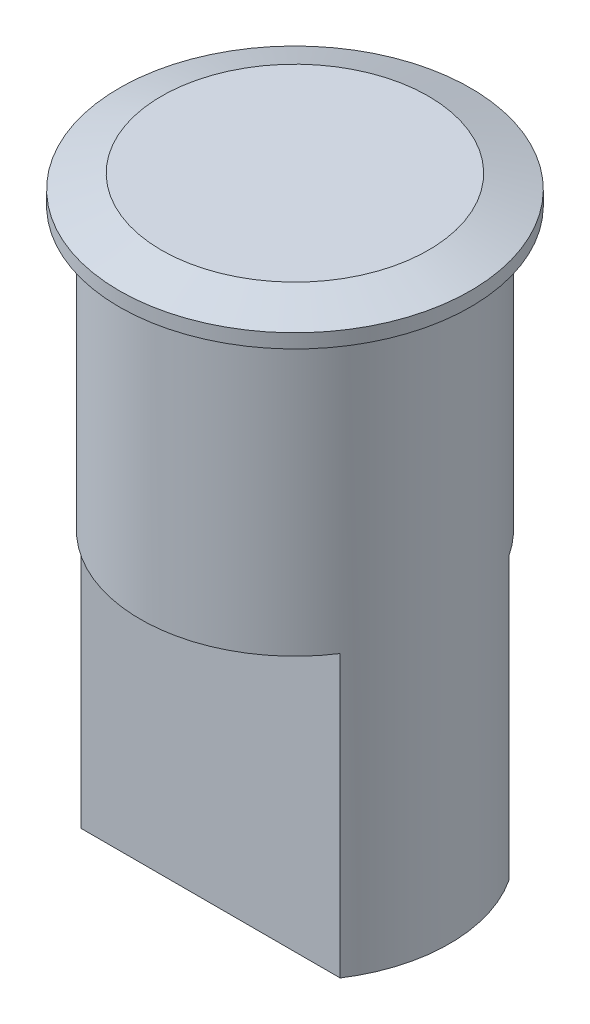
from build123d import *
from build123d.topology import SkipClean

# Parameters (mm, degrees)
SKETCH_1_R      = 11
EXTRUDE_1_DEPTH = 20
EXTRUDE_START   = 20
SKETCH_2_W      = 18.439088914
SKETCH_2_H      = 12
EXTRUDE_2_DEPTH = 20
SKETCH_3_R      = 12.5
EXTRUDE_3_DEPTH = 2
CHAMFER_1_SIZE  = 1
CHAMFER_1_SIZE2 = 3


with BuildPart() as part:
    # 草图1 → 凸台-拉伸1 (new body)
    with BuildSketch(Plane(origin=(0, 0, 0), x_dir=(1, 0, 0), z_dir=(0, 1, 0))):
        with Locations(Location((0, 0, 0), (0, 0, 270))):
            Circle(SKETCH_1_R)
    extrude(amount=EXTRUDE_1_DEPTH)

    # 草图2 → 凸台-拉伸2 (add)
    with SkipClean():  # the faces are left unmerged after this step: merging them gives an invalid solid
        with BuildSketch(Plane.XZ.offset(EXTRUDE_START)):
            with BuildLine():
                Line((-9.219544457, -6), (-9.219544457, 6))
                ThreePointArc((-9.219544457, 6), (-11, 0), (-9.219544457, -6))
            make_face()
            Rectangle(SKETCH_2_W, SKETCH_2_H)
            with BuildLine():
                ThreePointArc((11, 0), (10.545496409, 3.129297922), (9.219544457, 6))
                Line((9.219544457, 6), (9.219544457, -6))
                ThreePointArc((9.219544457, -6), (10.545496409, -3.129297922), (11, 0))
            make_face()
        extrude(amount=-EXTRUDE_2_DEPTH)

    # 草图3 → 凸台-拉伸3 (add)
    with SkipClean():  # the faces are left unmerged after this step: merging them gives an invalid solid
        with BuildSketch(Plane(origin=(0, 20, 0), x_dir=(1, 0, 0), z_dir=(0, 1, 0))):
            with Locations(Location((0, 0, 0), (0, 0, 270))):
                Circle(SKETCH_3_R)
        extrude(amount=EXTRUDE_3_DEPTH)

    # 倒角1
    chamfer_1_edges = [part.edges().sort_by_distance(p)[0] for p in [
        (0, 22, -12.5),
    ]]
    chamfer_1_side = [part.faces().sort_by_distance(p)[0] for p in [
        (0, 21, -12.5),
    ]]
    chamfer(chamfer_1_edges, length=CHAMFER_1_SIZE, length2=CHAMFER_1_SIZE2, reference=chamfer_1_side[0])


solid = part.part
